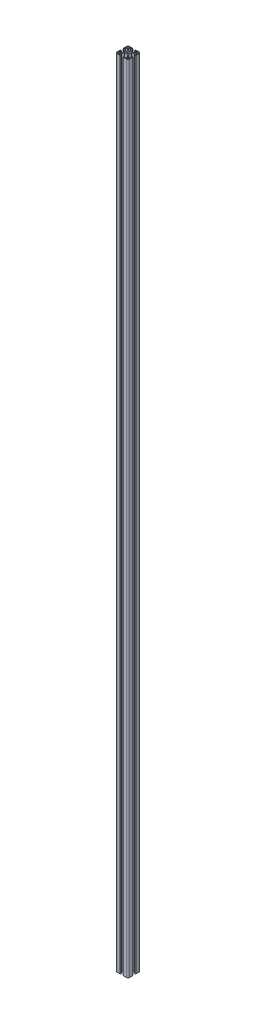
SolidWorks part; units mm, degrees
ref_plane "前视基准面" through (0, 0, 0) normal (0, 0, 1) x (1, 0, 0)
ref_plane "上视基准面" through (0, 0, 0) normal (0, 1, 0) x (1, 0, 0)
ref_plane "右视基准面" through (0, 0, 0) normal (1, 0, 0) x (0, 0, -1)
sketch "草图1" plane through (0, 0, 0) normal (1, 0, 0) x (0, 0, -1)
  line L0 (0, 0) -> (0, 2550)
  dimension "D1" = 2550
other "铝型材 40 X 40L X R4.5(1)"
ref_plane "基准面1" through (0, 0, 0) normal (0, 1, 0) x (0, 0, 1)
sketch "Sketch1" plane through (0, 0, 0) normal (0, 1, 0) x (0, 0, 1)
  line L0 (-5.1, 20) -> (-5.1, 19.5)
  line L1 (-5.1, 19.5) -> (-4.1, 19.5)
  line L2 (-4.1, 19.5) -> (-4.1, 17)
  line L3 (-6.1, 18.5) -> (-10.3, 18.5)
  line L4 (-15.5, -20) -> (-5.1, -20)
  line L5 (-20, -15.5) -> (-20, -5.1)
  line L6 (15.5, 20) -> (5.1, 20)
  line L7 (20, 15.5) -> (20, 5.1)
  line L8 (0, 14.8756) -> (0, 0) construction
  line L9 (0, 0) -> (14.1675, 0) construction
  line L10 (-10.3, 18.5) -> (-10.3, 11.3)
  line L11 (-10.3, 11.3) -> (-5, 6)
  line L12 (-5, 6) -> (5, 6)
  line L13 (10.3, 11.3) -> (5, 6)
  line L14 (10.3, 18.5) -> (10.3, 11.3)
  line L15 (6.1, 18.5) -> (10.3, 18.5)
  line L16 (4.1, 19.5) -> (4.1, 17)
  line L17 (5.1, 19.5) -> (4.1, 19.5)
  line L18 (5.1, 20) -> (5.1, 19.5)
  line L19 (-5.1, 20) -> (-15.5, 20)
  line L20 (20, 5.1) -> (19.5, 5.1)
  line L21 (11.8, 17.5) -> (15, 17.5)
  line L22 (11.8, 17.5) -> (11.8, 11.8)
  line L23 (11.8, 11.8) -> (17.5, 11.8)
  line L24 (17.5, 15) -> (17.5, 11.8)
  line L25 (19.5, 5.1) -> (19.5, 4.1)
  line L26 (19.5, 4.1) -> (17, 4.1)
  line L27 (17, 6.1) -> (17, 4.1)
  line L28 (18.5, 6.1) -> (17, 6.1)
  line L29 (18.5, 6.1) -> (18.5, 10.3)
  line L30 (18.5, 10.3) -> (11.3, 10.3)
  line L31 (11.3, 10.3) -> (6, 5)
  line L32 (6, 5) -> (6, -5)
  line L33 (11.3, -10.3) -> (6, -5)
  line L34 (18.5, -10.3) -> (11.3, -10.3)
  line L35 (18.5, -6.1) -> (18.5, -10.3)
  line L36 (18.5, -6.1) -> (17, -6.1)
  line L37 (17, -4.1) -> (17, -6.1)
  line L38 (19.5, -4.1) -> (17, -4.1)
  line L39 (19.5, -5.1) -> (19.5, -4.1)
  line L40 (20, -5.1) -> (19.5, -5.1)
  line L41 (5.1, -20) -> (5.1, -19.5)
  line L42 (5.1, -19.5) -> (4.1, -19.5)
  line L43 (4.1, -19.5) -> (4.1, -17)
  line L44 (6.1, -17) -> (4.1, -17)
  line L45 (6.1, -18.5) -> (6.1, -17)
  line L46 (6.1, -18.5) -> (10.3, -18.5)
  line L47 (10.3, -18.5) -> (10.3, -11.3)
  line L48 (10.3, -11.3) -> (5, -6)
  line L49 (5, -6) -> (-5, -6)
  line L50 (-10.3, -11.3) -> (-5, -6)
  line L51 (-10.3, -18.5) -> (-10.3, -11.3)
  line L52 (-6.1, -18.5) -> (-10.3, -18.5)
  line L53 (-6.1, -18.5) -> (-6.1, -17)
  line L54 (-4.1, -17) -> (-6.1, -17)
  line L55 (-4.1, -19.5) -> (-4.1, -17)
  line L56 (-5.1, -19.5) -> (-4.1, -19.5)
  line L57 (-5.1, -20) -> (-5.1, -19.5)
  line L58 (-20, -5.1) -> (-19.5, -5.1)
  line L59 (5.1, -20) -> (15.5, -20)
  line L60 (-20, 5.1) -> (-20, 15.5)
  line L61 (-19.5, -5.1) -> (-19.5, -4.1)
  line L62 (-6.1, 18.5) -> (-6.1, 17)
  line L63 (-6.1, 17) -> (-4.1, 17)
  line L64 (6.1, 18.5) -> (6.1, 17)
  line L65 (4.1, 17) -> (6.1, 17)
  line L66 (-19.5, -4.1) -> (-17, -4.1)
  line L67 (-15, 17.5) -> (-11.8, 17.5)
  line L68 (-17.5, 15) -> (-17.5, 11.8)
  line L69 (-17.5, 11.8) -> (-11.8, 11.8)
  line L70 (-11.8, 17.5) -> (-11.8, 11.8)
  line L71 (-17, -6.1) -> (-17, -4.1)
  line L72 (-18.5, -6.1) -> (-17, -6.1)
  line L73 (-18.5, -6.1) -> (-18.5, -10.3)
  line L74 (-18.5, -10.3) -> (-11.3, -10.3)
  line L75 (-11.3, -10.3) -> (-6, -5)
  line L76 (-6, -5) -> (-6, 5)
  line L77 (-11.3, 10.3) -> (-6, 5)
  line L78 (-18.5, 10.3) -> (-11.3, 10.3)
  line L79 (-18.5, 6.1) -> (-18.5, 10.3)
  line L80 (-18.5, 6.1) -> (-17, 6.1)
  line L81 (-17, 4.1) -> (-17, 6.1)
  line L82 (-19.5, 4.1) -> (-17, 4.1)
  line L83 (-19.5, 5.1) -> (-19.5, 4.1)
  line L84 (-20, 5.1) -> (-19.5, 5.1)
  line L85 (20, -5.1) -> (20, -15.5)
  line L87 (-17.5, -11.8) -> (-11.8, -11.8)
  line L88 (-17.5, -11.8) -> (-17.5, -15)
  line L89 (-15, -17.5) -> (-11.8, -17.5)
  line L90 (-11.8, -11.8) -> (-11.8, -17.5)
  line L91 (11.8, -11.8) -> (17.5, -11.8)
  line L92 (11.8, -11.8) -> (11.8, -17.5)
  line L93 (11.8, -17.5) -> (15, -17.5)
  line L94 (17.5, -11.8) -> (17.5, -15)
  circle A0 centre (0, 0) radius 3.4
  arc A1 (-20, 15.5) -> (-15.5, 20) centre (-15.5, 15.5) cw
  arc A2 (20, 15.5) -> (15.5, 20) centre (15.5, 15.5) ccw
  arc A3 (-15.5, -20) -> (-20, -15.5) centre (-15.5, -15.5) cw
  arc A4 (15.5, -20) -> (20, -15.5) centre (15.5, -15.5) ccw
  arc A5 (-15, 17.5) -> (-17.5, 15) centre (-15, 15) ccw
  arc A6 (17.5, 15) -> (15, 17.5) centre (15, 15) ccw
  arc A7 (17.5, -15) -> (15, -17.5) centre (15, -15) cw
  arc A8 (-17.5, -15) -> (-15, -17.5) centre (-15, -15) ccw
  point P2 (0, 10)
  point P4 (0, 0)
  point P5 (-20, -20)
  point P6 (20, -20)
  point P7 (20, 20)
  point P8 (-20, 20)
  point P36 (-20, 20)
  point P39 (20, 20)
  point P121 (0, 0)
  dimension "D1" = 20.6
  dimension "D2" = 40
  dimension "D3" = 8.2
  dimension "D4" = 10.2
  dimension "D5" = 14
  dimension "D6" = 6.8
  dimension "D7" = 4.5
  dimension "D8" = 45
  dimension "D12" = 2.5
  dimension "D13" = 5.7
  dimension "D14" = 1.5
  dimension "D18" = 2.5
  dimension "D19" = 2.5
  dimension "D15" = 2.5
  dimension "D9" = 0.5
  dimension "D10" = 1.5
  dimension "D11" = 10
  dimension "D16" = 3
  dimension "D17" = 2
  dimension "D20" = 1.5
  dimension "D21" = 2.5
